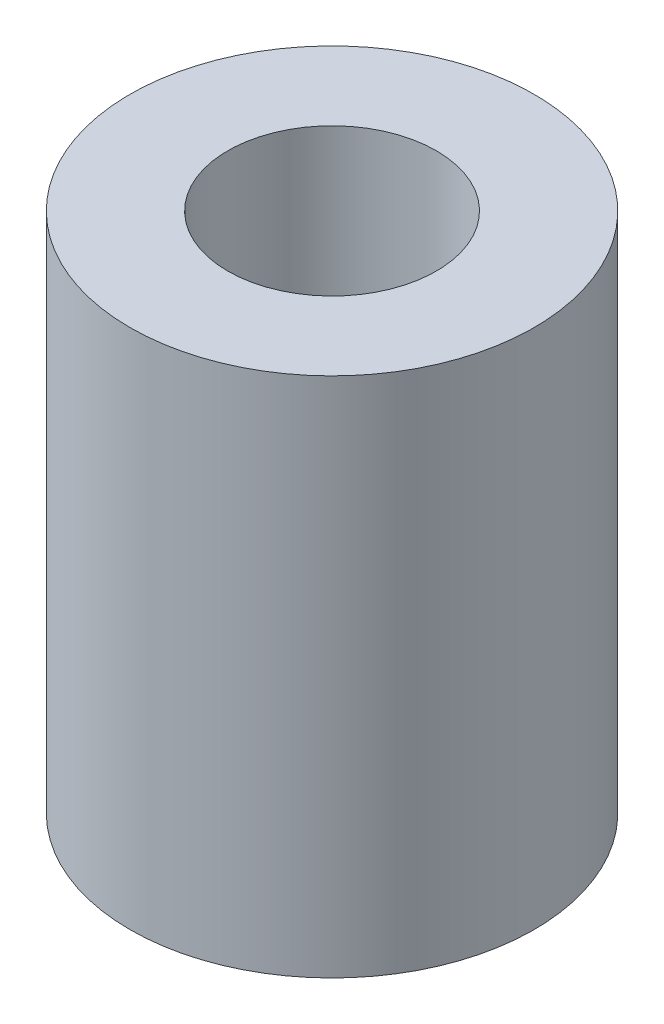
SolidWorks part; units mm, degrees
material "尼龙 101"
ref_plane "前视基准面" through (0, 0, 0) normal (0, 0, 1) x (1, 0, 0)
ref_plane "上视基准面" through (0, 0, 0) normal (0, 1, 0) x (1, 0, 0)
ref_plane "右视基准面" through (0, 0, 0) normal (1, 0, 0) x (0, 0, -1)
other "Configuration Table"
sketch "草图1" plane through (0, 0, 0) normal (0, 1, 0) x (1, 0, 0)
  circle A0 centre (0, 0) radius 1.6
  circle A1 centre (0, 0) radius 3.1
  dimension "D1" = 3.2
  dimension "D2" = 1.5
extrude "凸台-拉伸1" add sketch "草图1" along normal blind 8
